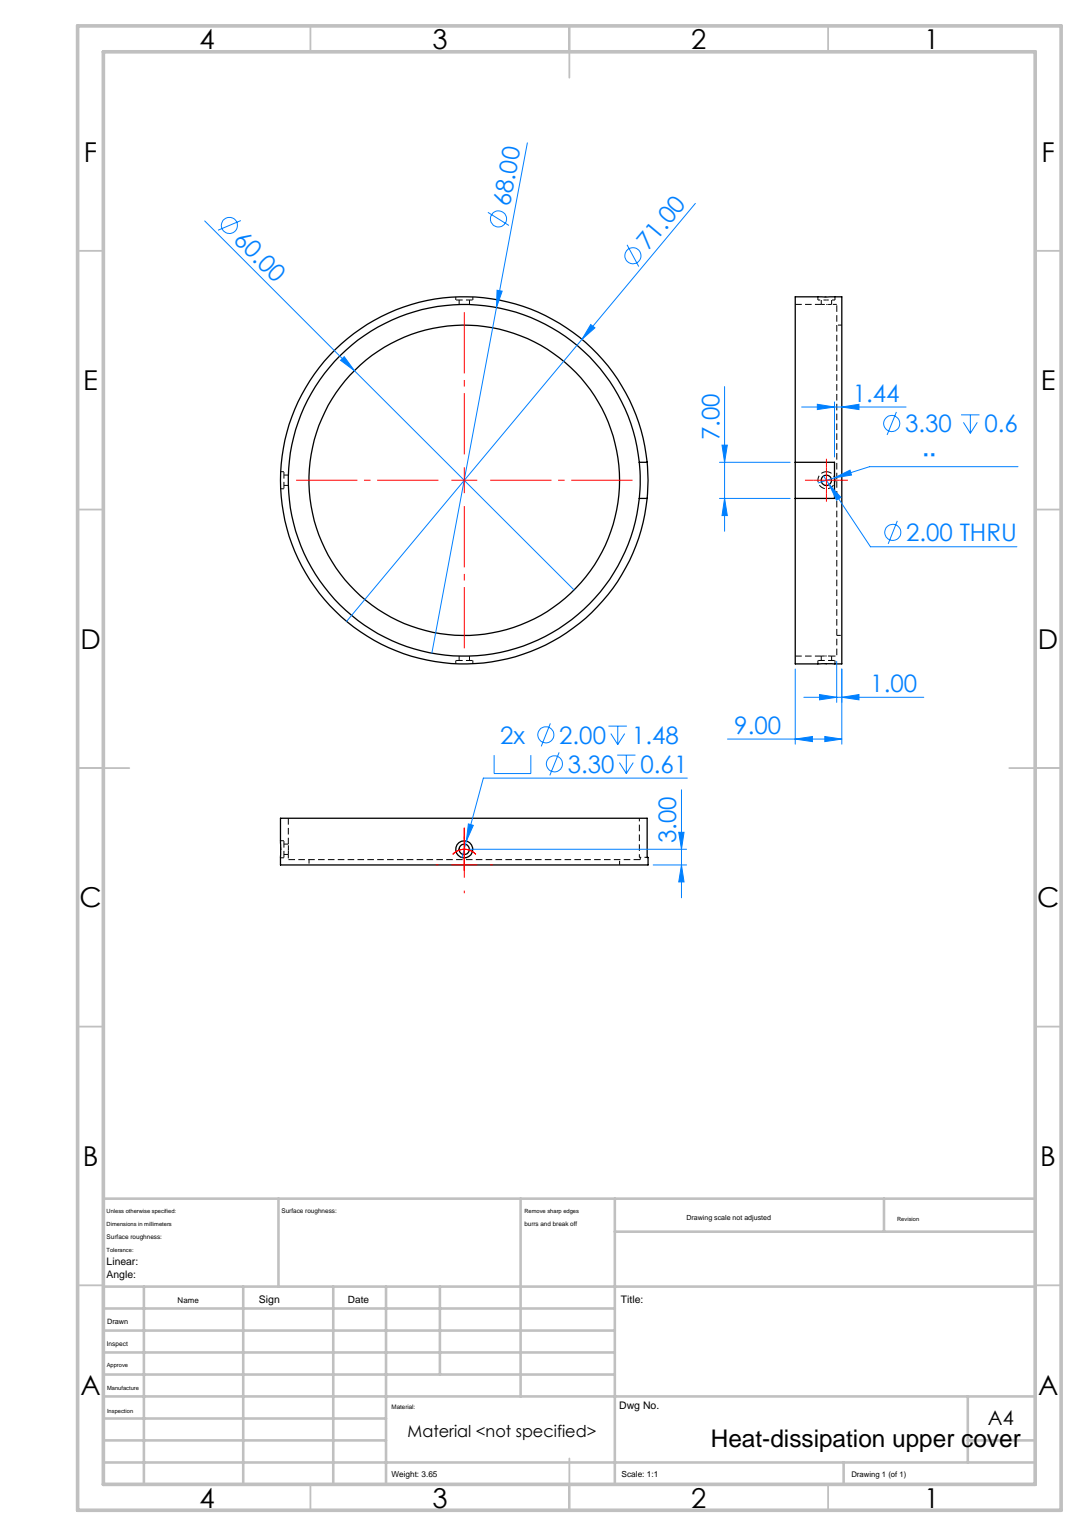
from build123d import *

# Parameters (mm, degrees)
SKETCH2_W          = 7
SKETCH2_H          = 10
CUT_EXTRUDE1_DEPTH = 52.004901725
CUT_EXTRUDE2_START = 34.85
SKETCH3_R          = 1.65
CUT_EXTRUDE2_DEPTH = 10.65
CIRPATTERN1_COUNT  = 4
SKETCH4_R          = 1
CUT_EXTRUDE3_DEPTH = 52.004901895
CIRPATTERN3_COUNT  = 4


with BuildPart() as part:
    # Sketch1 → Revolve1 (revolve)
    with BuildSketch(Plane.XY, mode=Mode.PRIVATE) as revolve1_sk:
        Polygon((34, 0), (34, 8), (30, 8), (30, 9), (35.5, 9), (35.5, 0), align=None)
    revolve(revolve1_sk.sketch.rotate(Axis((0, -1.347881032, 0), (0, 1, 0)), 90), axis=Axis((0, -1.347881032, 0), (0, 1, 0)))

    # Sketch2 → Cut-Extrude1 (cut, through all)
    with BuildSketch(Plane.XY):
        with Locations((0, 2.56)):
            Rectangle(SKETCH2_W, SKETCH2_H)
    extrude(amount=-CUT_EXTRUDE1_DEPTH, mode=Mode.SUBTRACT)

    # Sketch3 → Cut-Extrude2 (cut)
    with BuildSketch(Plane.XY.offset(CUT_EXTRUDE2_START)):
        with Locations(Location((0, 6, 0), (0, 0, 180))):
            Circle(SKETCH3_R)
    cut_extrude2 = extrude(amount=CUT_EXTRUDE2_DEPTH, mode=Mode.SUBTRACT)

    # CirPattern1: Cut-Extrude2 ×4 about axis, 1 skipped
    cirpattern1_axis = Axis((0, 0, 0), (0, -1, 0))
    add([cut_extrude2.rotate(cirpattern1_axis, i * 360 / CIRPATTERN1_COUNT) for i in range(1, CIRPATTERN1_COUNT) if i not in (2,)], mode=Mode.SUBTRACT)

    # Sketch4 → Cut-Extrude3 (cut, through all)
    with BuildSketch(Plane.XY):
        with Locations(Location((0, 6, 0), (0, 0, 180))):
            Circle(SKETCH4_R)
    cut_extrude3 = extrude(amount=CUT_EXTRUDE3_DEPTH, mode=Mode.SUBTRACT)

    # CirPattern3: Cut-Extrude3 ×4 about axis, 1 skipped
    cirpattern3_axis = Axis((0, -1.347881032, 0), (0, -1, 0))
    add([cut_extrude3.rotate(cirpattern3_axis, i * 360 / CIRPATTERN3_COUNT) for i in range(1, CIRPATTERN3_COUNT) if i not in (2,)], mode=Mode.SUBTRACT)


solid = part.part
